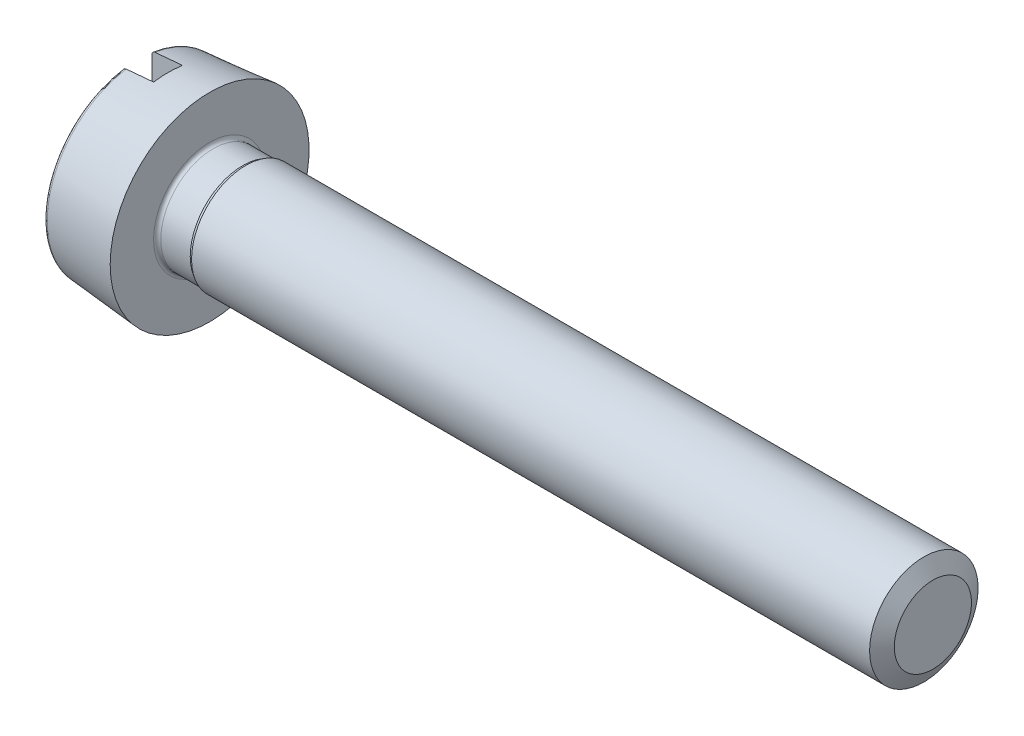
SolidWorks part; units mm, degrees
revolve "Base-Revolve" add sketch "Sketch1" angle 360 about L0
sketch "Sketch1" plane through (0, 0, 0) normal (0, 0, 1) x (1, 0, 0)
  line L0 (0, 0) -> (22, 0) construction
  line L1 (0, 0) -> (0, 2.4834)
  line L2 (2, 2.75) -> (0.0913, 2.583)
  line L3 (2, 2.75) -> (2, 1.55)
  line L4 (2.1, 1.45) -> (2.9134, 1.45)
  line L5 (2.9134, 1.45) -> (3, 1.5)
  line L6 (3, 1.5) -> (22, 1.5)
  line L7 (22, 1.5) -> (22, 0)
  line L8 (0, 0) -> (22, 0)
  arc A0 (2.1, 1.45) -> (2, 1.55) centre (2.1, 1.55) cw
  arc A1 (0, 2.4834) -> (0.0913, 2.583) centre (0.1, 2.4834) cw
cosmetic thread "Cosmetic Thread1" parameters "D1"=3.3866, "D2"=1.2
ref_plane "Front Plane" through (0, 0, 0) normal (0, 0, 1) x (1, 0, 0)
ref_plane "Top Plane" through (0, 0, 0) normal (0, 1, 0) x (1, 0, 0)
ref_plane "Right Plane" through (0, 0, 0) normal (1, 0, 0) x (0, 0, -1)
sketch "Dimension Sketch" plane through (0, 0, 0) normal (0, 0, 1) x (1, 0, 0)
  line L0 (0, 0) -> (22, 0)
  point P3 (0.85, 0)
  point P4 (1, 0)
  point P5 (3, 0)
  point P6 (5.5, 0)
  point P7 (0.8, 0)
  point P8 (3.1989, 0)
  point P9 (3.656, 0)
  point P10 (4.0948, 0)
  point P11 (21.5, 0)
  point P12 (21.9, 0)
  point P13 (2, 0)
sketch "Sketch2" plane through (0, 0, 0) normal (-1, 0, 0) x (0, 0, 1)
  line L0 (0, 0) -> (0, -1.8809) construction
  line L3 (0.4, 2.7208) -> (0.4, -2.7208)
  line L5 (-0.4, 2.7208) -> (-0.4, -2.7208)
  circle A1 centre (0, 0) radius 2.75 construction
  arc A2 (0.4, 2.7208) -> (-0.4, 2.7208) centre (0, 0) ccw
  arc A3 (-0.4, -2.7208) -> (0.4, -2.7208) centre (0, 0) ccw
extrude "Cut-Extrude1" cut sketch "Sketch2" against normal blind 0.85
sketch "Sketch3" plane through (0, 0, 0) normal (0, 1, 0) x (1, 0, 0)
  line L0 (21.75, 1.5) -> (22.25, 1.5)
  line L2 (22.25, 1.5) -> (22, 1.067)
  line L3 (22, 1.067) -> (21.75, 1.5)
  line L4 (22, -1.6037) -> (22, 3.368) construction
  line L10 (22, -1.5) -> (22, 1.5) construction
  line L11 (0, 0) -> (7.2232, 0) construction
revolve "Cut-Revolve1" cut sketch "Sketch3" angle 360 about L11
pattern_linear "LPattern1" [suppressed] count 39 along (1, 0, 0)
equation "\"l@Sketch1\" = \"l@Dimension Sketch\" "
equation "\"a@Sketch1\" = \"a@Dimension Sketch\" "
equation "\"r@Sketch1\" = \"r@Dimension Sketch\" "
equation "\"d@Sketch1\" = \"d@Dimension Sketch\" "
equation "\"k@Sketch1\" = \"k@Dimension Sketch\" "
equation "\"dk@Sketch1\" = \"dk@Dimension Sketch\" "
equation "\"n@Sketch2\" = \"n@Dimension Sketch\" "
equation "\"t@Cut-Extrude1\" = \"t@Dimension Sketch\" "
equation "\"D2@Sketch3\" = \"p@Dimension Sketch\" * 0.866"
equation "\"D3@Sketch3\" = \"d@Sketch1\" / 2"
equation "\"D1@Sketch1\" = \"d@Sketch1\" - \"r@Sketch1\""
equation "\"D1@LPattern1\" =  ( \"l@Sketch1\" - \"a@Sketch1\" )  / \"p@LPattern1\" + 1"
